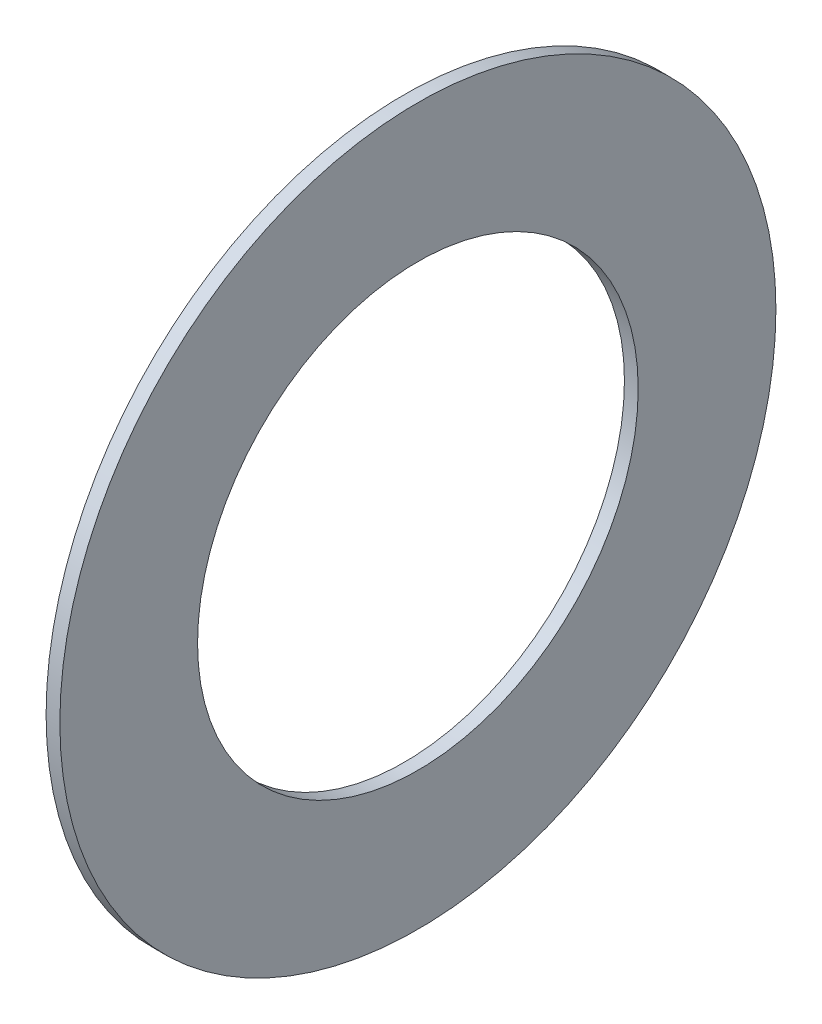
SolidWorks part; units mm, degrees
ref_plane "Front Plane" through (0, 0, 0) normal (0, 0, 1) x (1, 0, 0)
ref_plane "Top Plane" through (0, 0, 0) normal (0, 1, 0) x (1, 0, 0)
ref_plane "Right Plane" through (0, 0, 0) normal (1, 0, 0) x (0, 0, -1)
sketch "Sketch1" plane through (0, 0, 0) normal (1, 0, 0) x (0, 0, -1)
  circle A0 centre (0, 0) radius 8
  circle A1 centre (0, 0) radius 13
  dimension "D1" = 26
  dimension "D2" = 16
extrude "Boss-Extrude1" add sketch "Sketch1" along normal blind 0.5
